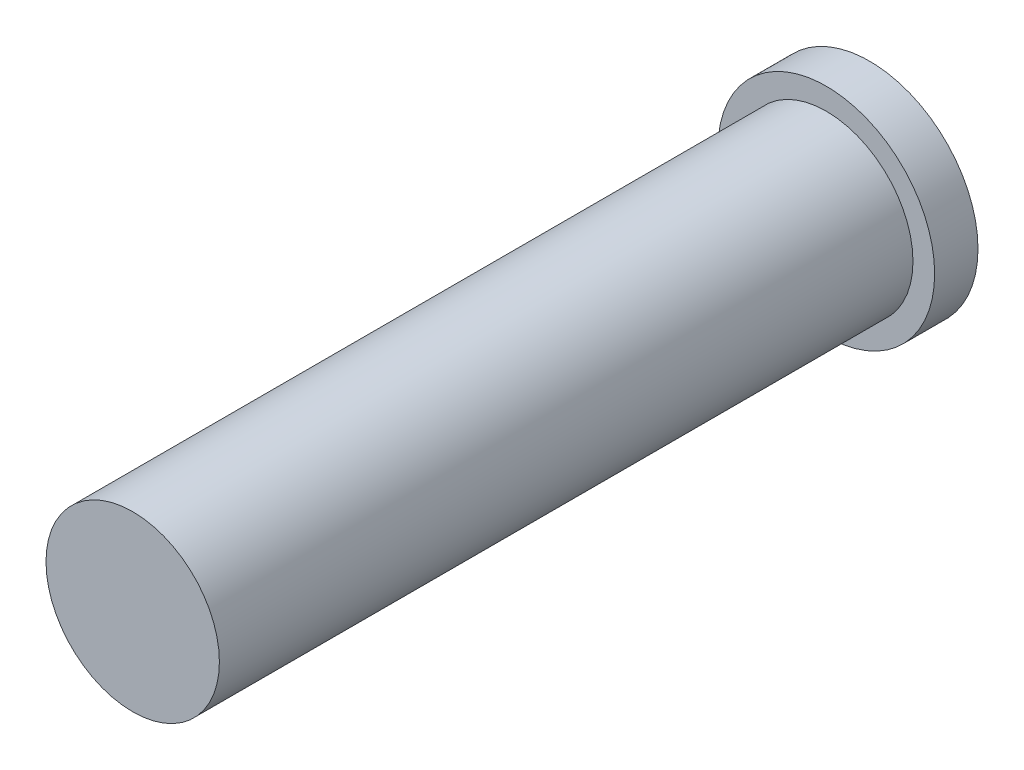
from build123d import *

# Parameters (mm, degrees)
SKETCH_1_R      = 2.5
EXTRUDE_1_DEPTH = 1
SKETCH_2_R      = 2
EXTRUDE_2_DEPTH = 16


with BuildPart() as part:
    # 草图1 → 凸台-拉伸1 (new body)
    with BuildSketch(Plane.XY):
        Circle(SKETCH_1_R)
    extrude(amount=EXTRUDE_1_DEPTH)

    # 草图2 → 凸台-拉伸2 (add)
    with BuildSketch(Plane.XY.offset(1)):
        Circle(SKETCH_2_R)
    extrude(amount=EXTRUDE_2_DEPTH)


solid = part.part
